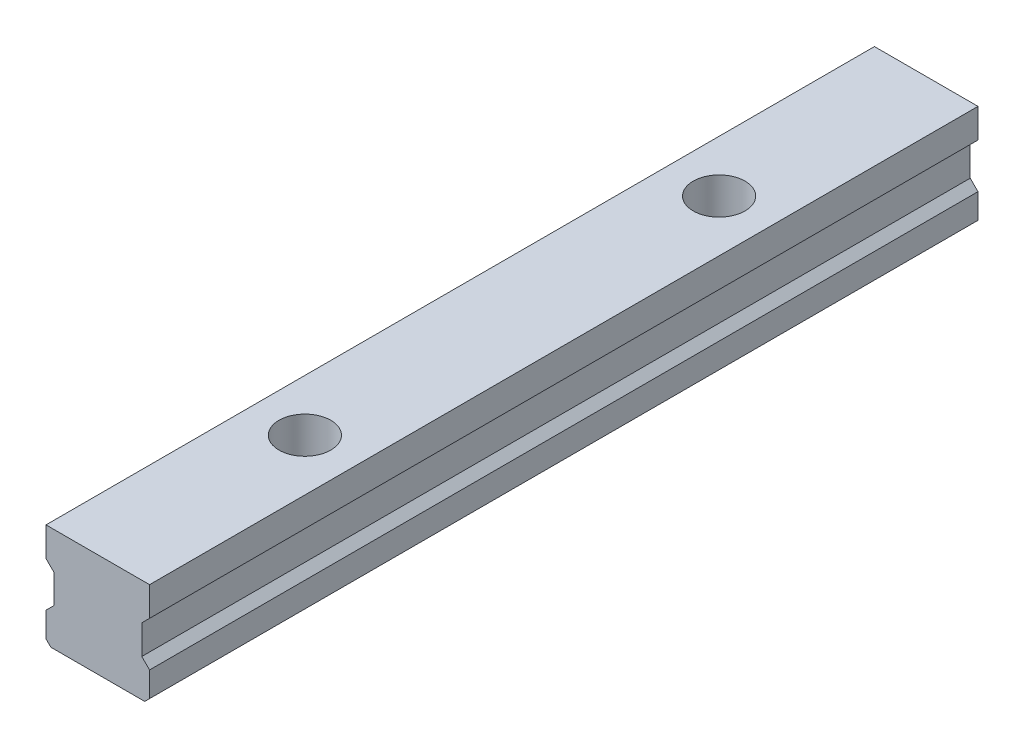
from build123d import *

# Parameters (mm, degrees)
EXTRUDE_1_DEPTH        = 50
CHAMFER_1_SIZE         = 0.7
PATTERN_LINEAR_1_COUNT = 2
PATTERN_LINEAR_1_PITCH = 60
MOVE_FACE_1_BY         = 10
MOVE_FACE_2_BY         = 10


with BuildPart() as part:
    # 草图1 → 凸台-拉伸1 (new, symmetric)
    with BuildSketch(Plane.XY):
        Polygon((-7.5, 0), (7.5, 0), (7.5, 4.3), (6.375, 5.425), (6.375, 9.65), (7.5, 10.775), (7.5, 15), (-7.5, 15), (-7.5, 10.775), (-6.375, 9.65), (-6.375, 5.425), (-7.5, 4.3), align=None)
    extrude(amount=EXTRUDE_1_DEPTH, both=True)

    # 倒角1
    chamfer_1_edges = [part.edges().sort_by_distance(p)[0] for p in [
        (7.5, 0, 0),
        (-7.5, 0, 0),
    ]]
    chamfer(chamfer_1_edges, length=CHAMFER_1_SIZE)

    # 草图3 → Cut-Revolve 1095 (revolve, cut)
    with BuildSketch(Plane(origin=(0, 0, 0), x_dir=(0, 0, -1), z_dir=(1, 0, 0)), mode=Mode.PRIVATE) as cut_revolve_1095_sk:
        Polygon((-30, 15), (-33.75, 15), (-33.75, 9.7), (-32.25, 9.7), (-32.25, 0), (-30, 0), align=None)
    cut_revolve_1095 = revolve(cut_revolve_1095_sk.sketch.rotate(Axis((0, 15, 30), (0, 1, 0)), 180), axis=Axis((0, 15, 30), (0, 1, 0)), mode=Mode.SUBTRACT)

    # 上锁孔阵列(线性)1: Cut-Revolve 1095 ×2
    with Locations(*[(0, 0, -i * PATTERN_LINEAR_1_PITCH) for i in range(1, PATTERN_LINEAR_1_COUNT)]):
        add(cut_revolve_1095, mode=Mode.SUBTRACT)

    # Move Face 1: a face moved outward by 10.0
    extrude(part.faces().sort_by_distance((0, 7.514633707, 50))[0], amount=MOVE_FACE_1_BY, dir=(0, 0, 1))

    # Move Face 2: a face moved outward by 10.0
    extrude(part.faces().sort_by_distance((0, 7.514633707, -50))[0], amount=MOVE_FACE_2_BY, dir=(0, 0, -1))


solid = part.part
